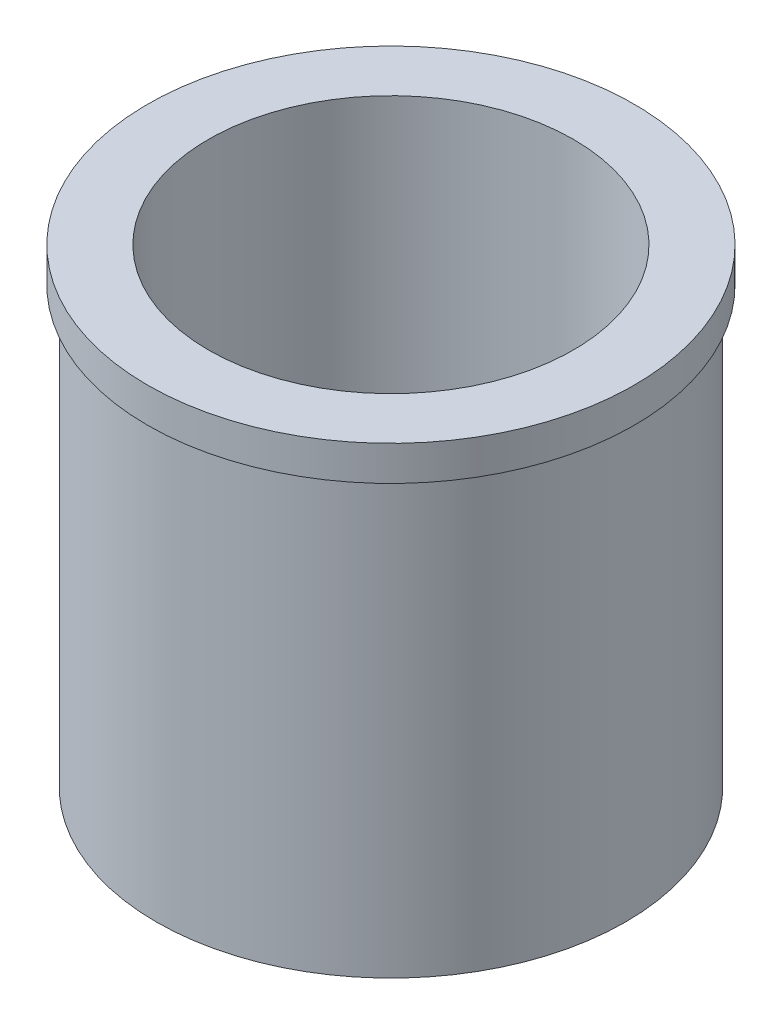
from build123d import *


with BuildPart() as part:
    # 草图1 → 旋转1 (revolve)
    with BuildSketch(Plane.XY, mode=Mode.PRIVATE) as revolve_1_sk:
        Polygon((10.5, 0), (14, 0), (14, -2), (13.5, -2), (13.5, -27), (10.5, -27), align=None)
    revolve(revolve_1_sk.sketch.rotate(Axis((0, 4.076999107, 0), (0, -1, 0)), 90), axis=Axis((0, 4.076999107, 0), (0, -1, 0)))


solid = part.part
